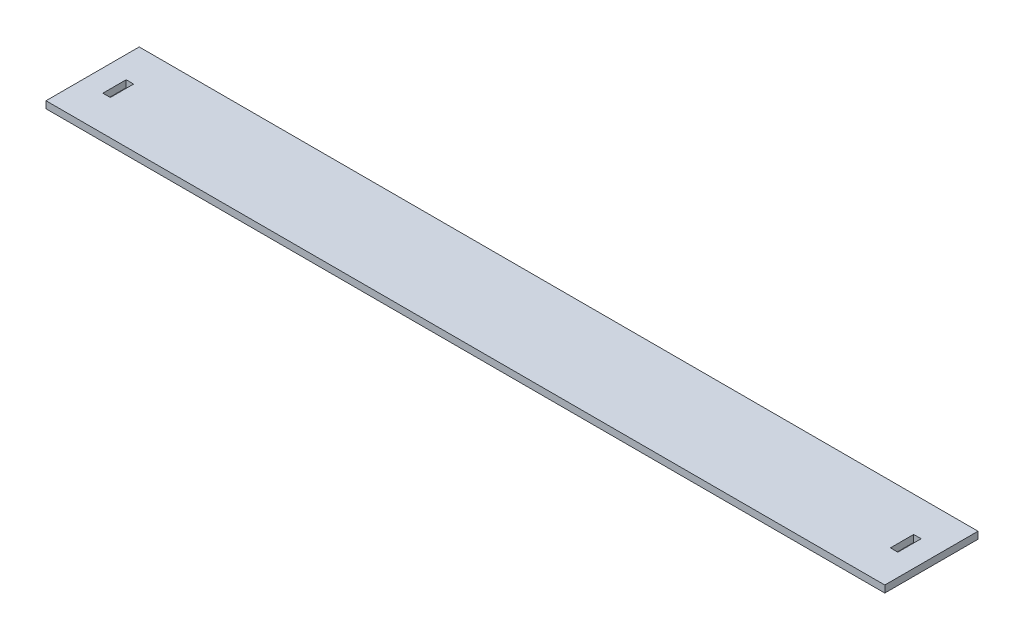
SolidWorks part; units mm, degrees
ref_plane "Front Plane" through (0, 0, 0) normal (0, 0, 1) x (1, 0, 0)
ref_plane "Top Plane" through (0, 0, 0) normal (0, 1, 0) x (1, 0, 0)
ref_plane "Right Plane" through (0, 0, 0) normal (1, 0, 0) x (0, 0, -1)
sketch "Sketch1" plane through (0, 0, 0) normal (0, 1, 0) x (1, 0, 0)
  line L1 (-180, -20) -> (180, -20)
  line L2 (-180, -20) -> (-180, 20)
  line L3 (-180, 20) -> (180, 20)
  line L4 (180, -20) -> (180, 20)
  line L5 (-180, -20) -> (180, 20) construction
  line L6 (-180, 20) -> (180, -20) construction
  point P0 (0, 0)
  dimension "D1" = 360
  dimension "D2" = 40
extrude "Boss-Extrude1" add sketch "Sketch1" along normal blind 3
sketch "Sketch2" plane through (0, 3, 0) normal (0, 1, 0) x (1, 0, 0)
  line L5 (-170.6, 5) -> (-167.4, 5)
  line L6 (-170.6, 5) -> (-170.6, -5)
  line L7 (-170.6, -5) -> (-167.4, -5)
  line L8 (-167.4, 5) -> (-167.4, -5)
  line L13 (-180, 20) -> (-180, -20) construction
  line L14 (-180, -20) -> (180, -20) construction
  line L15 (0, -1000) -> (0, 49000) construction
  line L16 (167.4, 5) -> (167.4, -5)
  line L17 (170.6, -5) -> (167.4, -5)
  line L18 (170.6, 5) -> (170.6, -5)
  line L19 (170.6, 5) -> (167.4, 5)
  point P9 (-167.4, 0)
  dimension "D1" = 10
  dimension "D2" = 3.2
  dimension "D3" = 9.4
  dimension "D4" = 20
extrude "Cut-Extrude1" cut sketch "Sketch2" against normal blind 10
